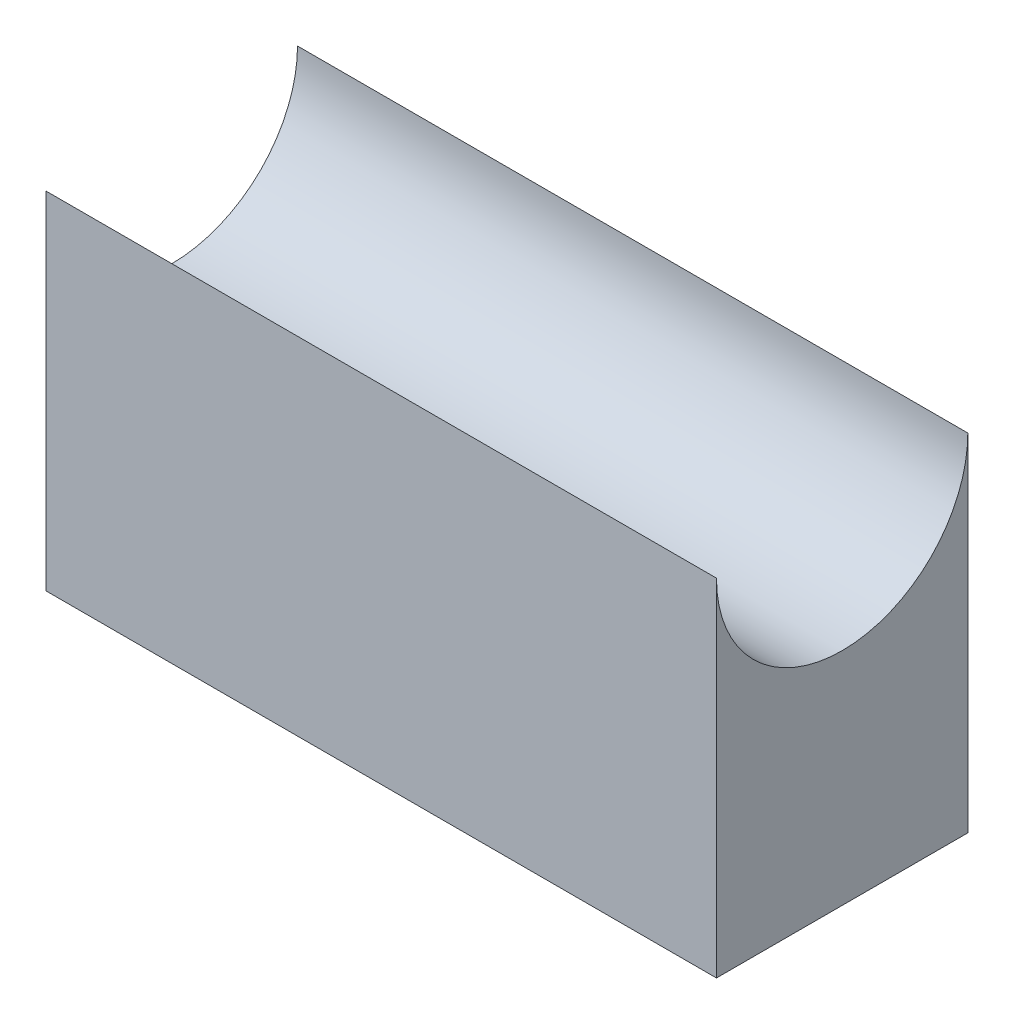
from build123d import *

# Parameters (mm, degrees)
SKETCH1_W           = 80
SKETCH1_H           = 30
BOSS_EXTRUDE1_DEPTH = 10
BOSS_EXTRUDE2_DEPTH = 80


with BuildPart() as part:
    # Sketch1 → Boss-Extrude1 (new body)
    with BuildSketch(Plane(origin=(0, 0, 0), x_dir=(1, 0, 0), z_dir=(0, 1, 0))):
        Rectangle(SKETCH1_W, SKETCH1_H)
    extrude(amount=BOSS_EXTRUDE1_DEPTH)

    # Sketch3 → Boss-Extrude2 (add)
    with BuildSketch(Plane.ZY.offset(40)):
        with BuildLine():
            Line((-15, 10), (-15, 41.330342273))
            ThreePointArc((-15, 41.330342273), (0, 26.330342273), (15, 41.330342273))
            Line((15, 41.330342273), (15, 10))
            Line((15, 10), (-15, 10))
        make_face()
    extrude(amount=-BOSS_EXTRUDE2_DEPTH)


solid = part.part
